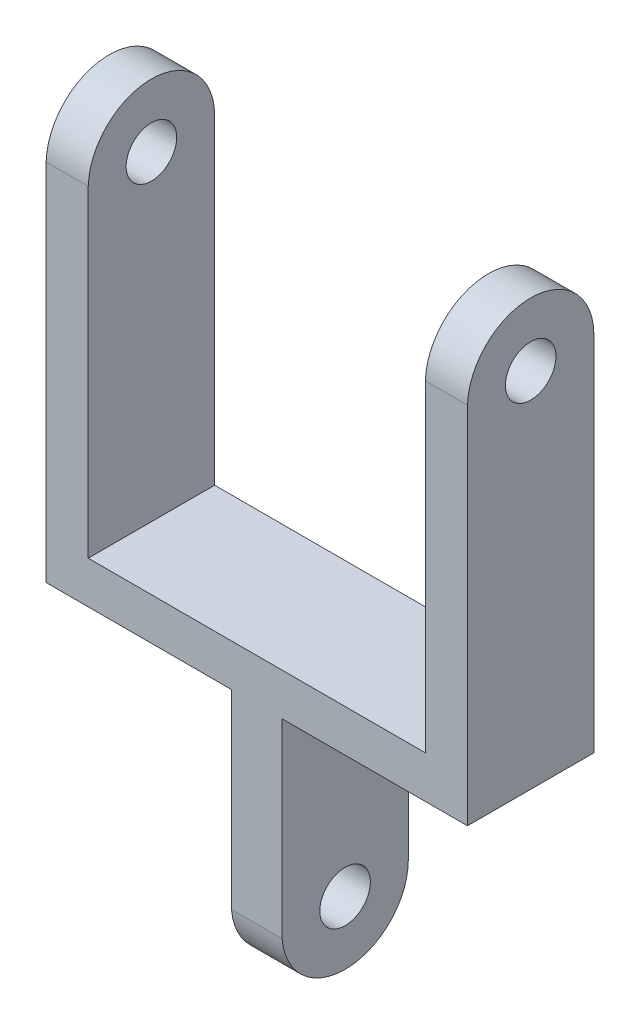
SolidWorks part; units mm, degrees
ref_plane "Front Plane" through (0, 0, 0) normal (0, 0, 1) x (1, 0, 0)
ref_plane "Top Plane" through (0, 0, 0) normal (0, 1, 0) x (1, 0, 0)
ref_plane "Right Plane" through (0, 0, 0) normal (1, 0, 0) x (0, 0, -1)
other "Configuration Table"
sketch "Sketch1" plane through (0, 0, 0) normal (0, 0, 1) x (1, 0, 0)
  line L0 (0, 0) -> (0, 164.9526) construction
  line L4 (20, 35) -> (-20, 35)
  line L5 (-20, 35) -> (-20, 85)
  line L6 (-20, 85) -> (-25, 85)
  line L7 (-25, 85) -> (-25, 30)
  line L8 (-25, 30) -> (-3, 30)
  line L9 (-3, 30) -> (-3, 0)
  line L10 (-3, 0) -> (0, 0)
  line L11 (3, 0) -> (0, 0)
  line L12 (3, 30) -> (3, 0)
  line L13 (25, 30) -> (3, 30)
  line L14 (25, 85) -> (25, 30)
  line L15 (20, 85) -> (25, 85)
  line L16 (20, 35) -> (20, 85)
  point P20 (0, 35)
  point P21 (0, 65)
  dimension "D1" = 85
  dimension "D3" = 6
  dimension "D4" = 40
  dimension "D5" = 50
  dimension "D6" = 5
  dimension "D7" = 50
extrude "Boss-Extrude1" add sketch "Sketch1" along normal blind 15
sketch "Sketch2" plane through (-25, 0, 0) normal (-1, 0, 0) x (0, 0, 1)
  line L0 (0.0032, 73) -> (-23.0887, 76.7199)
  line L1 (-23.0887, 76.7199) -> (-0.6618, 109.9617)
  line L2 (-0.6618, 109.9617) -> (34.9579, 90.5566)
  line L3 (34.9579, 90.5566) -> (15.0032, 73)
  line L4 (0.0236, 8) -> (-15.3016, 0.6071)
  line L5 (-15.3016, 0.6071) -> (-3.2806, -15.5924)
  line L6 (-3.2806, -15.5924) -> (32.4691, -12.3519)
  line L7 (32.4691, -12.3519) -> (24.8415, 4.3571)
  line L8 (24.8415, 4.3571) -> (15.0236, 8)
  line L9 (15, 0) -> (0, 0) construction
  circle A0 centre (7.5032, 73) radius 3
  circle A1 centre (7.5236, 8) radius 3
  arc A2 (15.0032, 73) -> (0.0032, 73) centre (7.5032, 73) ccw
  arc A3 (0.0236, 8) -> (15.0236, 8) centre (7.5236, 8) ccw
  dimension "D1" = 65
  dimension "D2" = 6
  dimension "D3" = 6
  dimension "D4" = 7.5
  dimension "D5" = 7.5
  dimension "D6" = 8
extrude "Cut-Extrude1" cut sketch "Sketch2" against normal through all
